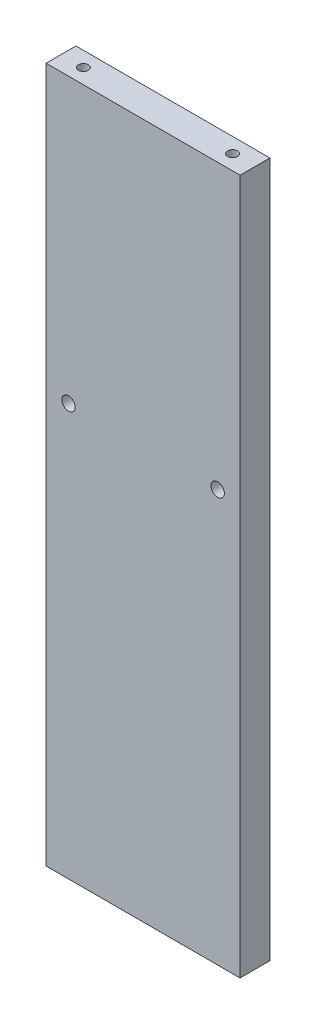
SolidWorks part; units mm, degrees
material "A6061"
ref_plane "前基準面" through (0, 0, 0) normal (0, 0, 1) x (1, 0, 0)
ref_plane "上基準面" through (0, 0, 0) normal (0, 1, 0) x (1, 0, 0)
ref_plane "右基準面" through (0, 0, 0) normal (1, 0, 0) x (0, 0, -1)
sketch "草图1" plane through (0, 0, 0) normal (0, 1, 0) x (1, 0, 0)
  line L1 (-32.5, 5) -> (32.5, 5)
  line L2 (-32.5, 5) -> (-32.5, -5)
  line L3 (-32.5, -5) -> (32.5, -5)
  line L4 (32.5, 5) -> (32.5, -5)
  line L5 (-32.5, 5) -> (32.5, -5) construction
  line L6 (-32.5, -5) -> (32.5, 5) construction
  point P0 (0, 0)
  dimension "D1" = 10
  dimension "D2" = 65
extrude "凸台-拉伸1" add sketch "草图1" along normal mid plane 233
sketch "草图2" plane through (0, 116.5, 0) normal (0, 1, 0) x (1, 0, 0)
  line L0 (0, 14.3945) -> (0, 0) construction
  point P0 (25, 0)
  point P13 (-25, 0)
  dimension "D1" = 50
hole_wizard "M4 螺纹孔1" positions "草图2" profile "草图3" tap size "M4" standard "GB"
sketch "草图3" plane through (25, 116.5, 0) normal (1, 0, 0) x (0, 0, 1)
  line L0 (0, 0) -> (0, 11.0914)
  line L1 (0, 11.0914) -> (1.65, 10.1)
  line L2 (1.65, 10.1) -> (1.65, 0)
  line L5 (1.65, 0) -> (0, 0)
  line L10 (0, 11.0914) -> (-1.65, 10.1) construction
  line L11 (0, -6.35) -> (0, 107.95) construction
  dimension "螺纹孔钻头直径" = 3.3
  dimension "螺纹孔钻头深度" = 10.1
  dimension "导头角度" = 118
cosmetic thread "孔螺纹线1" parameters "D1"=8, "D2"=4
cosmetic thread "孔螺纹线2" parameters "D1"=8, "D2"=4
mirror "镜向1" about plane through (0, 0, 0) normal (0, 1, 0) of "M4 螺纹孔1"
sketch "草图4" plane through (0, 0, -5) normal (0, 0, -1) x (-1, 0, 0)
  line L0 (0, 50.7126) -> (0, 0) construction
  line L2 (-32.5, -116.5) -> (32.5, -116.5) construction
  point P0 (25, 21.5)
  point P3 (-25, 21.5)
  dimension "D1" = 50
  dimension "D2" = 138
hole_wizard "M4 间隙孔1" positions "草图4" profile "草图5" hole size "M4" standard "GB" end condition through all
sketch "草图5" plane through (-25, 21.5, -5) normal (1, 0, 0) x (0, 1, 0)
  line L0 (0, 0) -> (0, 10)
  line L1 (0, 10) -> (2.25, 10)
  line L2 (2.25, 10) -> (2.25, 0)
  line L5 (2.25, 0) -> (0, 0)
  line L11 (0, -6.35) -> (0, 107.95) construction
  dimension "通孔孔直径" = 4.5
  dimension "通孔孔深度" = 10
